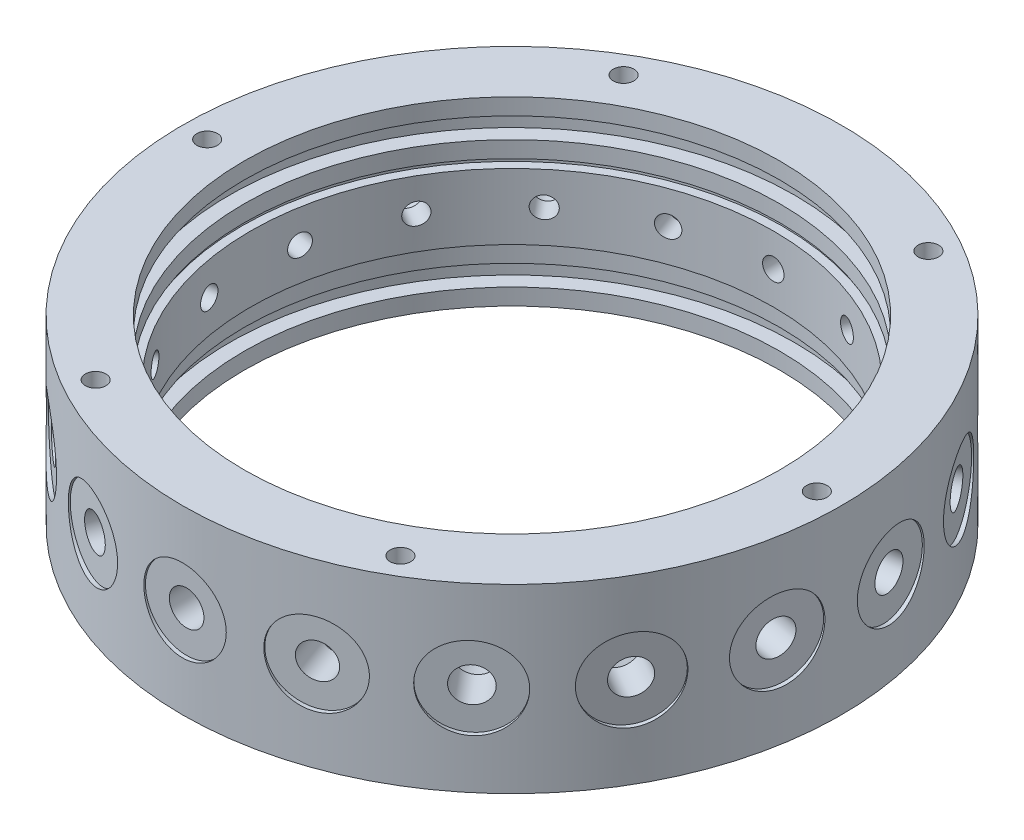
SolidWorks part; units mm, degrees
material "7075-T6 (SN)"
ref_plane "Front Plane" through (0, 0, 0) normal (0, 0, 1) x (1, 0, 0)
ref_plane "Top Plane" through (0, 0, 0) normal (0, 1, 0) x (1, 0, 0)
ref_plane "Right Plane" through (0, 0, 0) normal (1, 0, 0) x (0, 0, -1)
sketch "Sketch1" plane through (0, 0, 0) normal (0, 1, 0) x (1, 0, 0)
  circle A0 centre (0, 0) radius 40
  circle A1 centre (0, 0) radius 32.5
  dimension "D1" = 65
  dimension "D2" = 80
extrude "Boss-Extrude1" add sketch "Sketch1" along normal blind 22
sketch "Sketch2" plane through (0, 0, 0) normal (0, 0, 1) x (1, 0, 0)
  line L0 (0, 0) -> (0, 50000) construction
  line L1 (-43, 11) -> (49957, 11) construction
  line L2 (-40, 22) -> (-40, 0) construction
  line L3 (-32.5, 22) -> (-32.5, 0) construction
  line L4 (-30, 7) -> (-32.5, 7)
  line L5 (-30, 15) -> (-30, 7)
  line L6 (-30, 15) -> (-32.5, 15)
  line L7 (-32.5, 7) -> (-32.5, 15)
  line L8 (-30, 7) -> (-32.5, 15) construction
  line L9 (-30, 15) -> (-32.5, 7) construction
  point P7 (-40, 11)
  point P8 (-31.25, 11)
  dimension "D1" = 8
revolve "Revolve1" add sketch "Sketch2" angle 360 about L0
sketch "Sketch3" plane through (0, 0, 0) normal (0, 0, 1) x (1, 0, 0)
  line L0 (0, 0) -> (0, 50000) construction
  line L1 (-43, 11) -> (49957, 11) construction
  line L2 (-40, 22) -> (-40, 0) construction
  circle A0 centre (0, 11) radius 1.3
  point P7 (-40, 11)
  dimension "D1" = 2.6
extrude "Cut-Extrude1" cut sketch "Sketch3" against normal blind 53
pattern_circular "CirPattern1" count 18 over 360 about axis through (0, 22, 0) along (0, -1, 0) of "Cut-Extrude1"
ref_plane "Plane1" through (0, 0, 40) normal (0, 0, 1) x (1, 0, 0)
sketch "Sketch4" plane through (0, 0, 40) normal (0, 0, 1) x (1, 0, 0)
  circle A0 centre (0, 11) radius 5
  dimension "D1" = 10
extrude "Cut-Extrude2" cut sketch "Sketch4" against normal blind 0.5
pattern_circular "CirPattern2" count 18 over 360 about axis through (0, 0, 0) along (0, 1, 0) of "Cut-Extrude2"
hole_wizard "M5 Tapped Hole1" positions "3DSketch1" profile "Sketch5" tap size "M5" standard "Gb"
sketch3d "3DSketch1"
  line L0 (0, 11, 39.5) -> (0, 11, 29.9718) construction
  line L1 (0, 11, 39.5) -> (0, 11, 39.6863) construction
  point P0 (0, 11, 39.5)
  point P6 (0, 11, 39.5)
  point P8 (0, 11, 39.5)
  point P10 (0, 11, 39.5)
  point P12 (0, 11, 39.5)
  point P14 (0, 11, 39.5)
  point P16 (0, 11, 39.5)
sketch "Sketch5" plane through (0, 11, 39.5) normal (1, 0, 0) x (0, -1, 0)
  line L0 (0, 0) -> (0, 5.7618)
  line L1 (0, 5.7618) -> (2.1, 4.5)
  line L2 (2.1, 4.5) -> (2.1, 0)
  line L5 (2.1, 0) -> (0, 0)
  line L10 (0, 5.7618) -> (-2.1, 4.5) construction
  line L11 (0, -6.35) -> (0, 107.95) construction
  dimension "螺纹孔钻头直径" = 4.2
  dimension "螺纹孔钻头深度" = 4.5
  dimension "导头角度" = 118
cosmetic thread "Hole Thread 10" parameters "D1"=4.5, "D2"=5
cosmetic thread "Hole Thread 11" parameters "D1"=4.5, "D2"=5
cosmetic thread "Hole Thread 12" parameters "D1"=4.5, "D2"=5
cosmetic thread "Hole Thread 13" parameters "D1"=4.5, "D2"=5
cosmetic thread "Hole Thread 14" parameters "D1"=4.5, "D2"=5
cosmetic thread "Hole Thread 15" parameters "D1"=4.5, "D2"=5
cosmetic thread "Hole Thread 16" parameters "D1"=4.5, "D2"=5
pattern_circular "CirPattern3" count 18 over 360 about axis through (0, 22, 0) along (0, -1, 0) of "M5 Tapped Hole1"
sketch "Sketch6" plane through (0, 0, 0) normal (0, -1, 0) x (1, 0, 0)
  line L0 (0, 0) -> (50000, 0) construction
  line L1 (0, 0) -> (49240.3877, -8682.4089) construction
  circle A0 centre (0, 0) radius 37 construction
  circle A2 centre (35.7359, -9.5889) radius 0.5
  dimension "D1" = 74
  dimension "D4" = 1
  dimension "D3" = 10
extrude "Cut-Extrude3" cut sketch "Sketch6" against normal blind 2
hole_wizard "M3 Tapped Hole2" positions "3DSketch2" profile "Sketch7" tap size "M3" standard "Gb"
sketch3d "3DSketch2"
  line L1 (35.7359, 2, -9.5889) -> (35.7359, 0, -9.5889) construction
  point P4 (35.7359, 0, -9.5889)
sketch "Sketch7" plane through (35.7359, 0, -9.5889) normal (1, 0, 0) x (0, 0, -1)
  line L0 (0, 0) -> (0, 5.7511)
  line L1 (0, 5.7511) -> (1.25, 5)
  line L2 (1.25, 5) -> (1.25, 0)
  line L5 (1.25, 0) -> (0, 0)
  line L10 (0, 5.7511) -> (-1.25, 5) construction
  line L11 (0, -6.35) -> (0, 107.95) construction
  dimension "螺纹孔钻头直径" = 2.5
  dimension "螺纹孔钻头深度" = 5
  dimension "导头角度" = 118
cosmetic thread "Hole Thread 8" parameters "D1"=5, "D2"=3
pattern_circular "CirPattern4" count 6 over 360 about axis through (0, 0, 0) along (0, 1, 0) of "M3 Tapped Hole2"
sketch "Sketch8" plane through (0, 22, 0) normal (0, 1, 0) x (1, 0, 0)
  line L0 (0, 0) -> (-25000, 43301.2702) construction
  line L1 (0, 0) -> (0, 50000) construction
  circle A0 centre (-18.5, 32.0429) radius 0.5
  dimension "D1" = 1
  dimension "D3" = 37
  dimension "D2" = 30
extrude "Cut-Extrude4" cut sketch "Sketch8" against normal blind 3
hole_wizard "M3 Tapped Hole1" positions "3DSketch3" profile "Sketch9" tap size "M3" standard "Gb"
sketch3d "3DSketch3"
  line L0 (-18.5, 19, -32.0429) -> (-18.5, 22, -32.0429) construction
  point P0 (-18.5, 22, -32.0429)
sketch "Sketch9" plane through (-18.5, 22, -32.0429) normal (1, 0, 0) x (0, 0, 1)
  line L0 (0, 0) -> (0, 5.7511)
  line L1 (0, 5.7511) -> (1.25, 5)
  line L2 (1.25, 5) -> (1.25, 0)
  line L5 (1.25, 0) -> (0, 0)
  line L10 (0, 5.7511) -> (-1.25, 5) construction
  line L11 (0, -6.35) -> (0, 107.95) construction
  dimension "螺纹孔钻头直径" = 2.5
  dimension "螺纹孔钻头深度" = 5
  dimension "导头角度" = 118
cosmetic thread "Hole Thread 9" parameters "D1"=5, "D2"=3
pattern_circular "CirPattern5" count 6 over 360 about axis through (0, 0, 0) along (0, 1, 0) of "M3 Tapped Hole1"
sketch "Sketch12" plane through (0, 7, 0) normal (0, -1, 0) x (1, 0, 0)
  circle A0 centre (0, 0) radius 31.75
  dimension "D1" = 63.5
extrude "Cut-Extrude5" cut sketch "Sketch12" against normal blind 0.5
sketch "Sketch13" plane through (0, 15, 0) normal (0, 1, 0) x (1, 0, 0)
  circle A0 centre (0, 0) radius 31.75
  dimension "D1" = 63.5
extrude "Cut-Extrude6" cut sketch "Sketch13" against normal blind 44.5
sketch "Sketch16" plane through (0, 0, 0) normal (0, 0, 1) x (1, 0, 0)
  line L0 (0, 0) -> (0, 50000) construction
  line L1 (32.2269, 11) -> (50032.2269, 11) construction
  line L2 (32.5, 15) -> (-32.5, 15) construction
  line L3 (32.5, 15) -> (32.8, 15)
  line L4 (32.5, 15) -> (32.5, 15.5)
  line L5 (32.5, 15.5) -> (32.8, 15.5)
  line L6 (32.8, 15) -> (32.8, 15.5)
  line L7 (32.8, 7) -> (32.8, 6.5)
  line L8 (32.5, 6.5) -> (32.8, 6.5)
  line L9 (32.5, 7) -> (32.5, 6.5)
  line L11 (32.5, 7) -> (32.8, 7)
  dimension "D1" = 0.5
  dimension "D2" = 0.3
  dimension "D3" = 65
revolve "Cut-Revolve2" cut sketch "Sketch16" angle 360 about L0
sketch "Sketch17" plane through (0, 0, 0) normal (0, 0, 1) x (1, 0, 0)
  line L0 (0, 0) -> (0, 50000) construction
  line L1 (32.5, 18.75) -> (50032.5, 18.75) construction
  line L2 (32.5, 15.5) -> (32.5, 22) construction
  line L3 (32.5, 3.25) -> (50032.5, 3.25) construction
  line L4 (32.5, 0) -> (32.5, 6.5) construction
  line L6 (30.7, 4.5) -> (34.3, 4.5)
  line L7 (30.7, 4.5) -> (30.7, 2)
  line L8 (30.7, 2) -> (34.3, 2)
  line L9 (34.3, 4.5) -> (34.3, 2)
  line L10 (30.7, 4.5) -> (34.3, 2) construction
  line L11 (30.7, 2) -> (34.3, 4.5) construction
  line L12 (30.7, 20) -> (34.3, 20)
  line L13 (30.7, 20) -> (30.7, 17.5)
  line L14 (30.7, 17.5) -> (34.3, 17.5)
  line L15 (34.3, 20) -> (34.3, 17.5)
  line L16 (30.7, 20) -> (34.3, 17.5) construction
  line L17 (30.7, 17.5) -> (34.3, 20) construction
  point P7 (32.5, 18.75)
  point P9 (32.5, 3.25)
  point P12 (32.5, 3.25)
  point P18 (32.5, 18.75)
  dimension "D1" = 1.8
  dimension "D2" = 2.5
  dimension "D3" = 2.5
  dimension "D4" = 1.8
revolve "Cut-Revolve3" cut sketch "Sketch17" angle 360 about L0
ref_plane "Plane2" through (0, 11, 0) normal (0, 1, 0) x (1, 0, 0)
sketch "Sketch18" plane through (0, 0, 0) normal (0, -1, 0) x (1, 0, 0)
  line L0 (-30.1822, 21.4018) -> (40756.5164, -28899.9609) construction
  line L1 (0, 0) -> (50000, 0) construction
  line L2 (0, 0) -> (-35.7359, 9.5889) construction
  circle A0 centre (-30.1822, 21.4018) radius 1.5
  circle A1 centre (30.1822, -21.4018) radius 1.5
  circle A2 centre (0, 0) radius 37 construction
  dimension "D1" = 3
  dimension "D2" = 3
  dimension "D4" = 74
  dimension "D3" = 35.34
extrude "Cut-Extrude7" cut sketch "Sketch18" against normal blind 5
